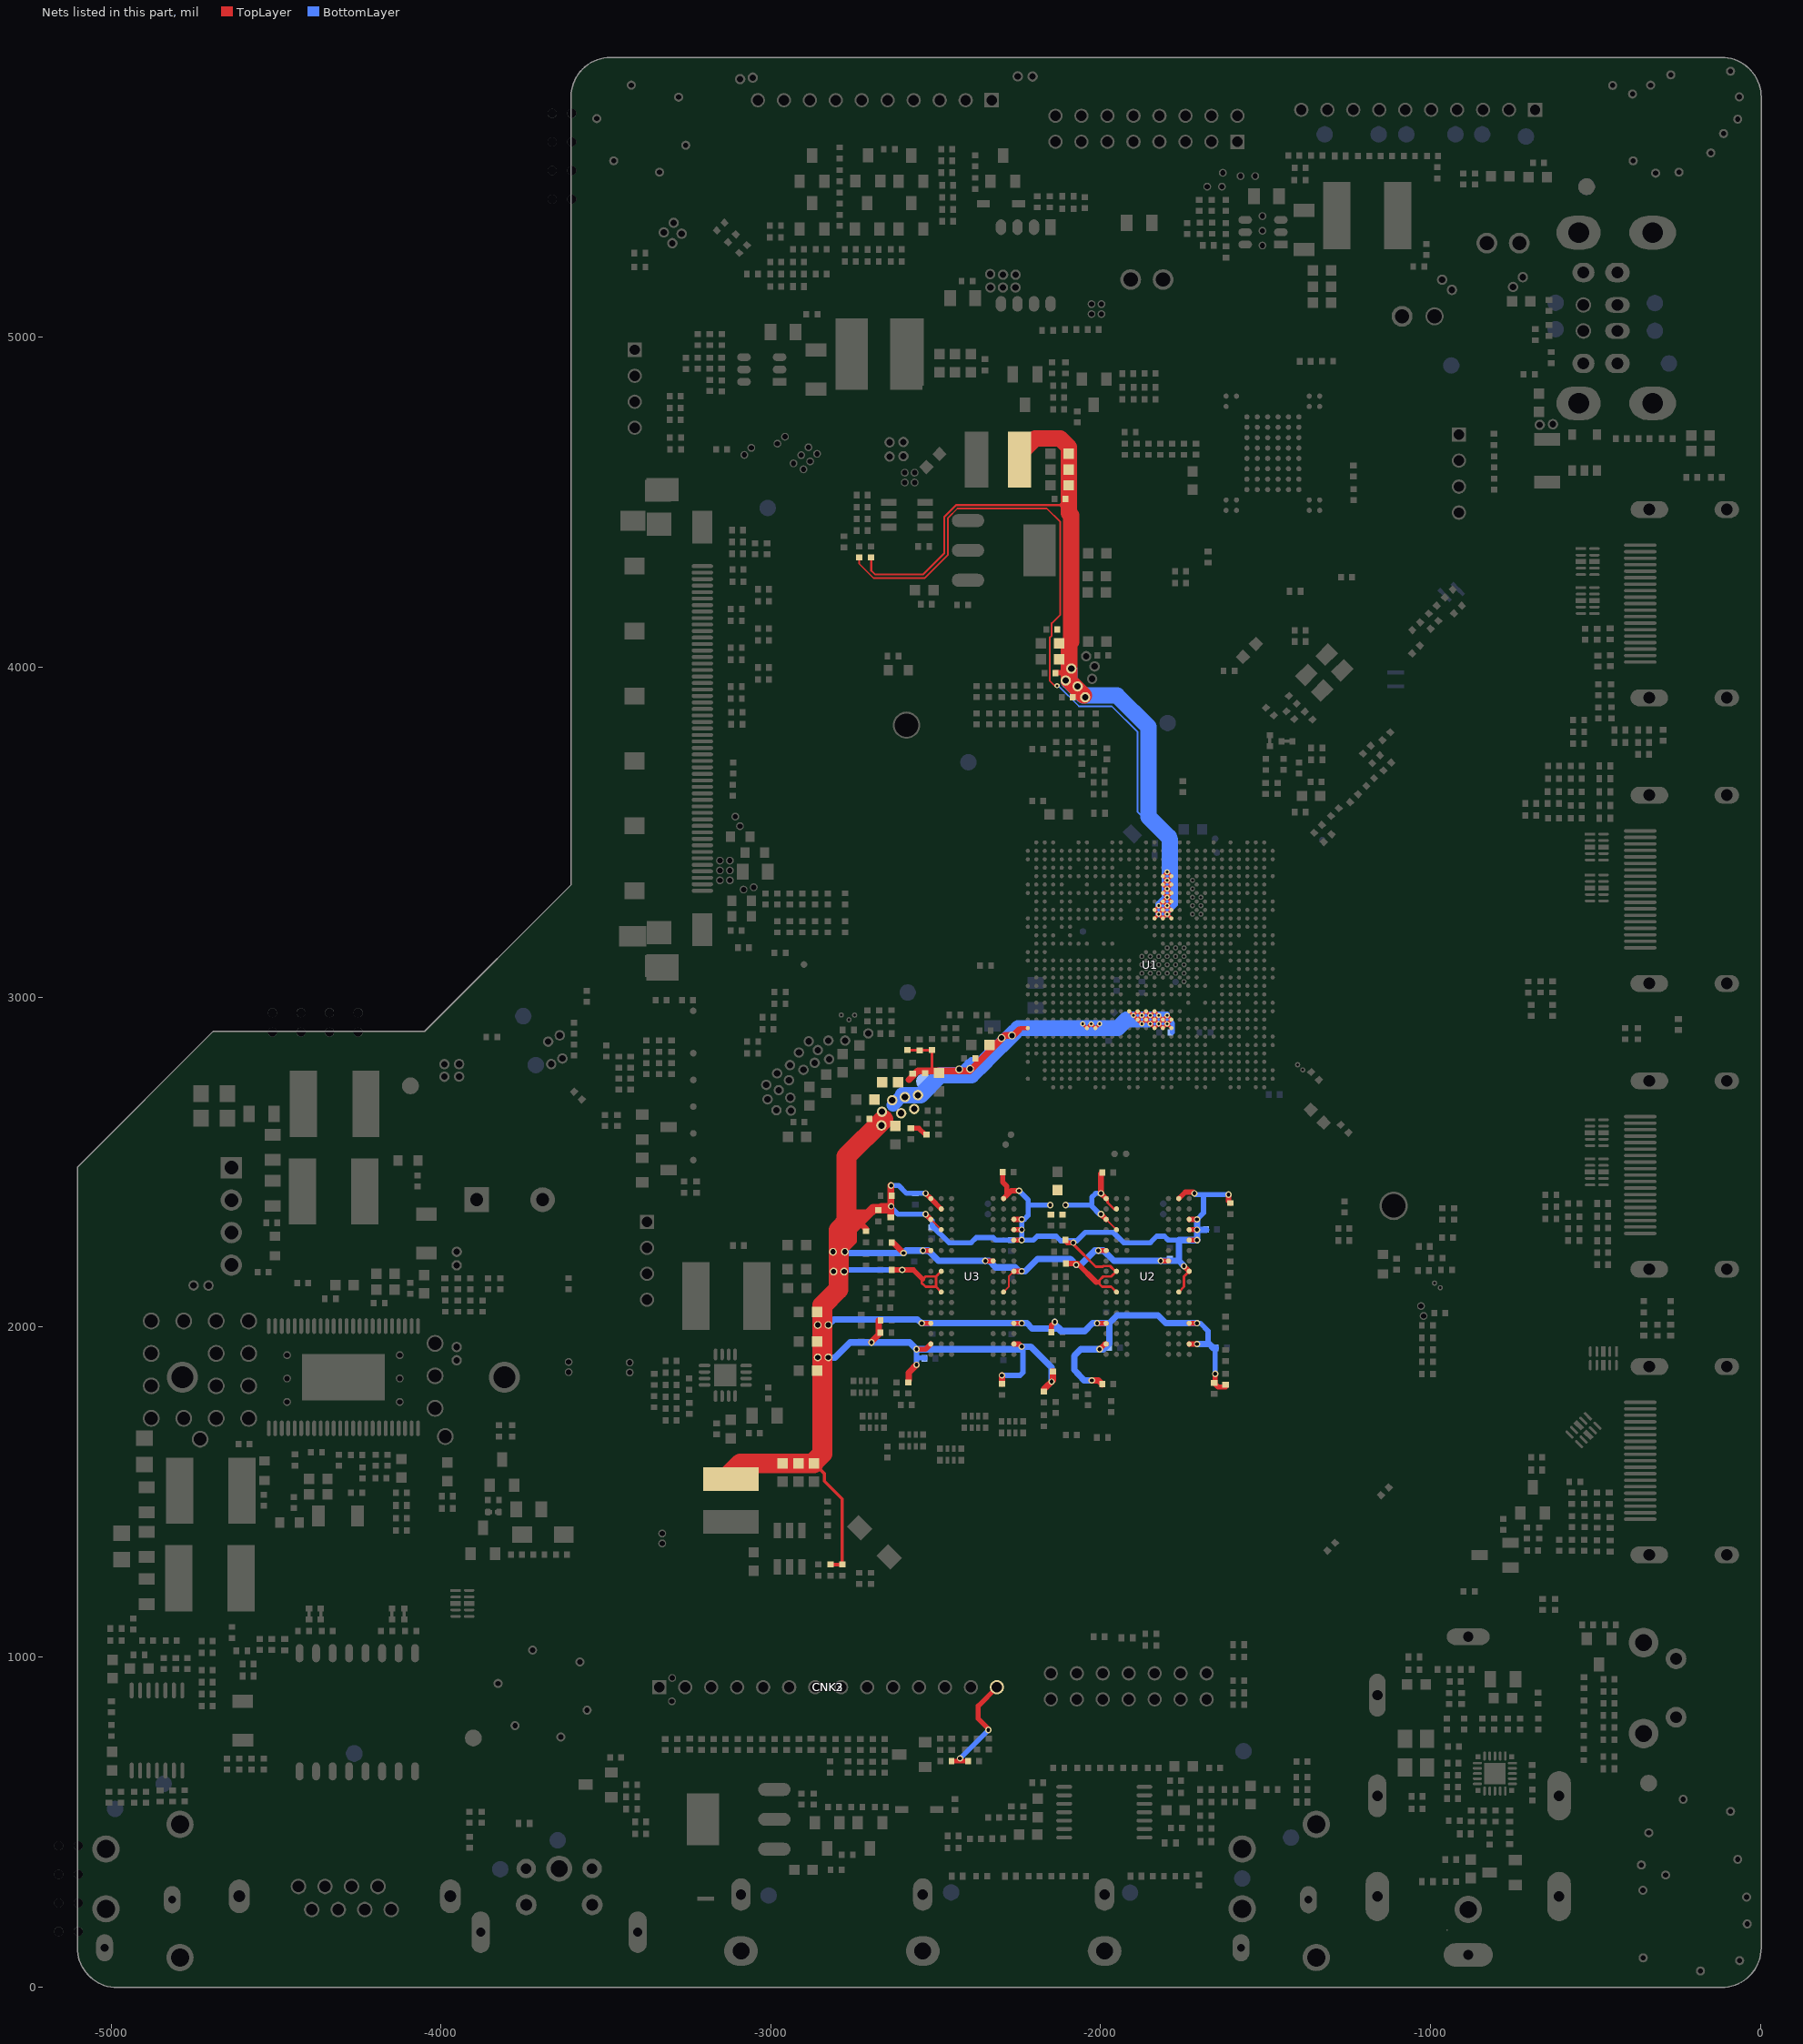
[diagram p0: the nets of this part, all layers, seen from the top]
# Altium PCB MISC86290.PcbDoc (part 8 of 31)
Units mil, origin at the board's own origin, x right, y up, seen from the top; angles counter-clockwise.
Board outline 5104.71 x 5851.49 mil, 2 copper layers (TopLayer, BottomLayer), stack 61.855 mil thick; 1026 components, 667 nets, 4280 pads, 2294 vias.

## Via types
v1: diameter 19.68, hole 11.81, TopLayer to BottomLayer, tented both sides, 1189 vias
v2: diameter 19.68/19.68 (per signal layer), hole 11.81, TopLayer to BottomLayer, tented both sides, 366 vias
v3: diameter 15.75, hole 7.87, TopLayer to BottomLayer, tented both sides, 348 vias
v4: diameter 23.62, hole 15.75, TopLayer to BottomLayer, tented both sides, 309 vias
v5: diameter 15.75/15.75 (per signal layer), hole 7.87, TopLayer to BottomLayer, tented both sides, 59 vias
v6: diameter 24/24 (per signal layer), hole 16, TopLayer to BottomLayer, tented both sides, 23 vias

## Nets (pads, with @x,y where several pads share a name; then routed paths per layer and width w, separated by ;. In a path a pad name is that pad's centre, name@x,y a point inside that pad or via, vN(x,y) a via of type N, cw(c..) or ccw(c..) an arc to the next point about the centre after c; other vN are vias at no path point) (continued)
0.95V_VDDCPU: C32.1 C33.1 C34.1 C35.2 C36.2 C209.1 C210.1 C211.1 CD53.2 CD54.2 CD55.2 CD56.2 LD51.2 pad.VIA5@-1798.54,3251.57 pad.VIA5@-1798.54,3277.17 pad.VIA5@-1798.54,3302.76 pad.VIA5@-1798.54,3328.35 pad.VIA5@-1798.54,3353.94 pad.VIA5@-1798.54,3379.53 pad.VIA5@-1824.13,3251.57 pad.VIA5@-1824.13,3277.17 pad.VIA5@-2047,3909 pad.VIA5@-2070,3942 pad.VIA5@-2089,3996 pad.VIA5@-2106,3960 RD53.2 RD60.1 U1.AA13 U1.AA14 U1.AA15 U1.AB13 U1.AB14 U1.AB15 U1.AC13 U1.AC14 U1.AD13 U1.AD14 U1.AE13 U1.AE14 U1.AF13 U1.AF14 | length 5527.1
  TopLayer w5: RD60.1@-2732.5,4333.04 -2732.5,4314.54 -2687.96,4270 -2534.42,4270 -2463,4341.42 -2463,4452.69 -2434.26,4481.43 -2163.43,4481.43 -2122.5,4440.5 -2122.5,4159.5 -2148.46,4133.54 -2148.46,4096.54 -2154,4091 -2154,3958 v3@-2140,3944
  TopLayer w6: RD53.2@-2695.5,4333.04 -2695.5,4293 -2683.5,4281 -2539.3,4281 -2474.4,4345.9 -2474.4,4456.02 -2438.64,4491.78 -2123.99,4491.78 ; CD53.2@-2101.91,4504.86 -2096.84,4509.92 ; CD53.2@-2101.91,4513.86 -2123.99,4491.78 ; -2096.84,4464.63 -2123.99,4491.78
  TopLayer w10: U1.AA15@-1836.93,3238.78 pad.VIA5@-1824.13,3251.57 ; U1.AA13@-1785.75,3238.78 pad.VIA5@-1798.54,3251.57 ; pad.VIA5@-1824.13,3251.57 U1.AB15@-1836.93,3264.37 pad.VIA5@-1824.13,3277.17 ; pad.VIA5@-1824.13,3251.57 U1.AA14@-1811.34,3238.78 pad.VIA5@-1798.54,3251.57 ; pad.VIA5@-1824.13,3251.57 U1.AB14@-1811.34,3264.37 ; pad.VIA5@-1824.13,3277.17 U1.AB14@-1811.34,3264.37 ; pad.VIA5@-1824.13,3277.17 U1.AC14@-1811.34,3289.96 ; U1.AB14@-1811.34,3264.37 pad.VIA5@-1798.54,3251.57 ; U1.AB14@-1811.34,3264.37 pad.VIA5@-1798.54,3277.17 ; U1.AC14@-1811.34,3289.96 pad.VIA5@-1798.54,3277.17 ; U1.AC14@-1811.34,3289.96 pad.VIA5@-1798.54,3302.76 ; pad.VIA5@-1798.54,3251.57 U1.AB13@-1785.75,3264.37 pad.VIA5@-1798.54,3277.17 ; pad.VIA5@-1798.54,3277.17 U1.AC13@-1785.75,3289.96 pad.VIA5@-1798.54,3302.76 ; pad.VIA5@-1798.54,3302.76 U1.AD13@-1785.75,3315.55 pad.VIA5@-1798.54,3328.35 ; pad.VIA5@-1798.54,3302.76 U1.AD14@-1811.34,3315.55 pad.VIA5@-1798.54,3328.35 ; pad.VIA5@-1798.54,3328.35 U1.AE13@-1785.75,3341.14 pad.VIA5@-1798.54,3353.94 ; pad.VIA5@-1798.54,3328.35 U1.AE14@-1811.34,3341.14 pad.VIA5@-1798.54,3353.94 ; pad.VIA5@-1798.54,3353.94 U1.AF13@-1785.75,3366.73 pad.VIA5@-1798.54,3379.53 U1.AF14@-1811.34,3366.73 pad.VIA5@-1798.54,3353.94
  TopLayer w17: C33.1@-2137.27,3984 -2120.45,3984 ; pad.VIA5@-2076.68,3941.77 pad.VIA5@-2066.23,3941.77
  TopLayer w50: LD51.2@-2246.24,4629.43 -2246.24,4645.79 -2198.03,4694 -2123,4694 -2096.84,4667.84 -2096.84,4509.92 -2096.84,4467.84 -2089.83,4460.83 -2089.83,4077.92 ; -2095.75,4072 -2095.75,3959.3 -2077.45,3941 -2074.23,3937.77 pad.VIA5@-2051.45,3915
  BottomLayer w5: v3@-2128.5,3944 -2066,3881.5 -1966.23,3881.5 -1888,3803.27 -1888,3561.28 -1875.62,3548.89 ; pad.VIA5@-1799.72,3278.03 pad.VIA5@-1799.27,3278.03
  BottomLayer w12: pad.VIA5@-1824.13,3254.03 -1822.93,3255.24 -1822.93,3277.17 -1822.93,3278.03 pad.VIA5@-1823.1,3278.2 ; pad.VIA5@-1800.13,3278.03 pad.VIA5@-1799.72,3278.03 ; pad.VIA5@-1799.27,3278.03 pad.VIA5@-1797.72,3278.03
  BottomLayer w15: pad.VIA5@-1798.54,3328.35 -1797.72,3327.53 -1797.72,3324.03 -1790.72,3324.03 -1773.22,3324.03 -1773.22,3281.03 -1794.72,3259.53
  BottomLayer w18: pad.VIA5@-1824.13,3251.57 pad.VIA5@-1799.72,3275.98 ; -1806.14,3299.12 pad.VIA5@-1806.14,3302.03 ; pad.VIA5@-1798.54,3379.53 -1806.14,3379.53 pad.VIA5@-1806.14,3302.03 ; pad.VIA5@-1793.68,3282.03 pad.VIA5@-1798.54,3277.17 pad.VIA5@-1799.72,3275.98 ; pad.VIA5@-1806.14,3302.03 -1799.72,3295.62 -1799.72,3278.03 -1799.72,3277.17 pad.VIA5@-1799.72,3275.98
  BottomLayer w20: pad.VIA5@-1823.1,3278.2 pad.VIA5@-1824.13,3277.17 ; -1806.14,3299.12 -1824.13,3281.12 pad.VIA5@-1824.13,3277.17 ; pad.VIA5@-1798.54,3251.57 pad.VIA5@-1824.13,3251.57 -1824.13,3254.03 pad.VIA5@-1824.13,3277.17 ; pad.VIA5@-1798.54,3277.17 -1799.72,3277.17 -1822.93,3277.17 pad.VIA5@-1824.13,3277.17
  BottomLayer w50: pad.VIA5@-2095.75,3995 -2095.75,3957.75 -2053,3915 -1951,3915 -1855,3819 -1855,3546.69 -1793.37,3485.06 ; -1790.72,3294.53 -1790.72,3324.03 -1790.72,3477.39
  other v3: -2132.5,3944
1V5_DDR: 1V5_DDR.1 C37.1 C38.1 C39.2 C40.2 C41.2 C42.1 C43.1 C44.2 C45.1 C46.2 C48.1 C50.1 C51.2 C58.2 C61.2 C62.2 C63.2 C64.2 C65.2 C66.2 C67.2 C68.2 C69.2 C70.2 C71.2 C73.2 C74.2 C75.2 C76.2 C77.2 C78.2 C79.2 C80.2 C81.2 C82.2 C83.2 C84.2 C85.2 C86.2 C87.2 C88.2 C89.2 C90.2 C91.2 C92.2 C93.2 C94.2 C95.2 C96.2 C206.1 C207.1 C208.1 CD23.2 CD25.2 CD26.2 CD27.2 LD21.2 pad.VIA5@-1798.54,2918.9 pad.VIA5@-1798.54,2944.49 pad.VIA5@-1824.13,2918.9 pad.VIA5@-1824.13,2944.49 pad.VIA5@-1849.72,2918.9 pad.VIA5@-1849.72,2944.49 pad.VIA5@-1875.32,2918.9 pad.VIA5@-1875.32,2944.49 pad.VIA5@-1900.91,2944.49 pad.VIA5@-2003.27,2918.9 pad.VIA5@-2028.86,2918.9 pad.VIA5@-2054.45,2918.9 pad.VIA5@-2269.02,2883.46 pad.VIA5@-2300.6,2876.14 pad.VIA5@-2396.1,2782.4 pad.VIA5@-2429,2781 pad.VIA5@-2554,2703.03 pad.VIA5@-2565.5,2661 pad.VIA5@-2593.5,2697 pad.VIA5@-2605,2648 pad.VIA5@-2632,2687.5 pad.VIA5@-2663,2652.5 pad.VIA5@-2665,2611 pad.VIA5@-2775.72,2228.03 pad.VIA5@-2777.72,2168.03 pad.VIA5@-2809.72,2168.03 pad.VIA5@-2811.72,2228.03 pad.VIA5@-2825.72,1908.03 pad.VIA5@-2825.72,2006.03 pad.VIA5@-2857.72,1908.03 pad.VIA5@-2857.72,2006.03 R44.2 R46.2 R63.2 R66.2 R101.2 R103.2 R107.2 R118.2 RD22.2 U1.H13 U1.H14 U1.H15 U1.H22 U1.H23 U1.H30 U1.J13 U1.J14 U1.J15 U1.J16 U1.J17 U1.K15 U1.K16 U1.K17 U1.K18 U2.A1 U2.A8 U2.B2 U2.C1 U2.C9 U2.D2 U2.D9 U2.E9 U2.F1 U2.G7 U2.H2 U2.H9 U2.K2 U2.K8 U2.N1 U2.N9 U2.R1 U2.R9 U3.A1 U3.A8 U3.B2 U3.C1 U3.C9 U3.D2 U3.D9 U3.E9 U3.F1 U3.G7 U3.H2 U3.H9 U3.K2 U3.K8 U3.N1 U3.N9 U3.R1 U3.R9 | length 13478.8
  TopLayer w3.94: U3.C1@-2515.08,2326.38 U3.D2@-2483.58,2294.88 ; U2.C1@-1983.58,2326.38 U2.D2@-1952.09,2294.88
  TopLayer w5: CD23.2@-2783.52,1279.73 CD23.2@-2783.25,1280 ; -2539.72,2144.25 -2539.43,2144.54 ; pad.VIA5@-2269.02,2883.46 pad.VIA5@-2269.02,2883.86 ; C82.2@-2107.28,2263.78 -2107.28,2261.42 C82.2@-2106.83,2260.96
  TopLayer w5.91: U3.K8@-2294.61,2105.91 -2278.86,2121.65 -2278.86,2153.15 U3.H9@-2263.11,2168.9
  TopLayer w7.87: -2539.72,2144.25 -2542.64,2141.34 -2542.64,2133.46 -2530.83,2121.65 -2499.33,2121.65 ; -2539.43,2144.54 -2530.83,2153.15 -2499.33,2153.15 ; U3.K2@-2483.58,2105.91 -2499.33,2121.65 ; U3.H2@-2483.58,2168.9 -2499.33,2153.15 ; v2(-2082.99,2255.51) -2082.01,2249.61 -2015.08,2182.68 -1993.43,2182.68 -1991.46,2184.65 -1971.77,2184.65 -1956.02,2168.9 U2.H2@-1952.09,2168.9 -1967.83,2153.15 -1992.44,2153.15 -2004.25,2141.34 -2004.25,2135.43 ; -2013.11,2135.43 -2004.25,2135.43 ; U2.A1@-1983.58,2389.37 -1979.65,2385.43 -1979.65,2377.56 -1959.96,2357.87 U2.B2@-1952.09,2357.87 ; U2.K2@-1952.09,2105.91 -1967.83,2121.65 -1995.39,2121.65 -2004.25,2130.51 -2004.25,2135.43 ; U2.K8@-1763.11,2105.91 -1747.36,2121.65 -1747.36,2153.15 U2.H9@-1731.61,2168.9 ; -2499.33,2121.65 -2499.33,2153.15
  TopLayer w8: C38.1@-2585.66,2839.58 R46.2@-2511.84,2839.58 -2511.84,2776.03 -2511.84,2775.6
  TopLayer w9.84: U1.H14@-1812.32,2907.09 U1.H14@-1811.34,2906.1 pad.VIA5@-1798.54,2918.9 U1.J13@-1785.75,2931.69
  TopLayer w10: CD27.2@-2869.29,1586.68 -2838,1555.4 -2838,1533 -2783.52,1478.52 CD23.2@-2783.52,1279.73 ; RD22.2@-2819.25,1279.73 CD23.2@-2783.52,1279.73 ; CD23.2@-2783.52,1278.74 CD23.2@-2783.52,1279.73 ; pad.VIA5@-2054.45,2918.9 U1.H23@-2041.65,2906.1 pad.VIA5@-2028.86,2918.9 U1.H22@-2016.06,2906.1 pad.VIA5@-2003.27,2918.9 ; U1.K18@-1913.7,2957.28 pad.VIA5@-1900.91,2944.49 ; U1.H14@-1812.32,2907.09 pad.VIA5@-1824.13,2918.9 ; U1.H13@-1785.75,2906.1 pad.VIA5@-1798.54,2918.9 -1806.2,2926.56 U1.J14@-1811.34,2931.69 ; U1.J13@-1785.75,2931.69 pad.VIA5@-1798.54,2944.49 U1.J14@-1811.34,2931.69 ; pad.VIA5@-1900.91,2944.49 U1.J17@-1888.11,2931.69 ; pad.VIA5@-1900.91,2944.49 U1.K17@-1888.11,2957.28 pad.VIA5@-1875.32,2944.49 ; U1.J17@-1888.11,2931.69 pad.VIA5@-1875.32,2944.49 ; U1.J17@-1888.11,2931.69 pad.VIA5@-1875.32,2918.9 U1.J16@-1862.52,2931.69 ; pad.VIA5@-1875.32,2944.49 U1.J16@-1862.52,2931.69 ; pad.VIA5@-1875.32,2944.49 U1.K16@-1862.52,2957.28 pad.VIA5@-1849.72,2944.49 ; U1.J16@-1862.52,2931.69 pad.VIA5@-1849.72,2944.49 ; U1.J16@-1862.52,2931.69 pad.VIA5@-1849.72,2918.9 ; pad.VIA5@-1849.72,2918.9 U1.H15@-1836.93,2906.1 pad.VIA5@-1824.13,2918.9 ; pad.VIA5@-1849.72,2918.9 U1.J15@-1836.93,2931.69 ; pad.VIA5@-1849.72,2944.49 U1.K15@-1836.93,2957.28 pad.VIA5@-1824.13,2944.49 ; pad.VIA5@-1849.72,2944.49 U1.J15@-1836.93,2931.69 ; U1.J15@-1836.93,2931.69 pad.VIA5@-1824.13,2918.9 ; U1.J15@-1836.93,2931.69 pad.VIA5@-1824.13,2944.49 ; pad.VIA5@-1824.13,2918.9 U1.J14@-1811.34,2931.69 ; pad.VIA5@-1824.13,2944.49 U1.J14@-1811.34,2931.69
  TopLayer w12: -2248.33,2900.43 -2242.65,2906.1 U1.H30@-2220.79,2906.1
  TopLayer w15: C77.2@-2575.5,2602.46 -2550.84,2602.46 -2531.41,2583.04 C48.1@-2528.5,2583.04
  TopLayer w15.75: C68.2@-2634.12,2172.83 v2(-2601.69,2172.83) -2567.72,2172.83 -2539.43,2144.54 ; v2(-2558.39,1932.68) -2530.83,1932.68 U3.R1@-2515.08,1948.43 ; v2(-2542.64,2011.42) U3.N1@-2515.08,2011.42 ; v2(-2538.7,2231.89) U3.F1@-2515.08,2231.89 ; v2(-2530.83,2342.13) U3.C1@-2515.08,2326.38 ; v2(-2530.83,2405.12) U3.A1@-2515.08,2389.37 U3.B2@-2483.58,2357.87 ; v2(-2349.72,2200.39) U3.G7@-2326.1,2200.39 ; C76.2@-2296.89,2470.08 -2296.97,2470 -2296.97,2438.98 -2284.76,2426.77 -2284.76,2399.21 ; U3.A8@-2294.61,2389.37 -2284.76,2399.21 ; U3.R9@-2263.11,1948.43 -2247.36,1948.43 v2(-2239.49,1940.55) ; U3.N9@-2263.11,2011.42 v2(-2239.49,2011.42) ; U3.H9@-2263.11,2168.9 v2(-2239.49,2168.9) ; U3.E9@-2263.11,2263.39 v2(-2239.49,2263.39) ; U3.D9@-2263.11,2294.88 v2(-2239.49,2294.88) ; U3.C9@-2263.11,2326.38 v2(-2239.49,2326.38) ; v2(-2247.36,2412.99) -2270.98,2412.99 -2284.76,2399.21 ; C81.2@-2149.25,1983.86 -2149.25,2005.2 v2(-2139.09,2015.35) ; C82.2@-2106.83,2260.96 -2101.38,2255.51 v2(-2082.99,2255.51) ; C73.2@-2105.32,2192.52 -2070.2,2192.52 -2013.11,2135.43 ; v2(-2011.14,2011.42) U2.N1@-1983.58,2011.42 ; v2(-2007.2,2231.89) U2.F1@-1983.58,2231.89 ; v2(-2003.27,1932.68) -1987.52,1948.43 U2.R1@-1983.58,1948.43 ; v2(-1999.33,2342.13) U2.C1@-1983.58,2326.38 ; v2(-1999.33,2405.12) U2.A1@-1983.58,2389.37 ; v2(-1818.23,2200.39) U2.G7@-1794.61,2200.39 ; U2.A8@-1763.11,2389.37 -1743.43,2409.06 -1719.8,2409.06 v2(-1715.87,2405.12) ; v2(-1747.36,2184.65) U2.H9@-1731.61,2168.9 ; U2.R9@-1731.61,1948.43 v2(-1707.99,1948.43) ; U2.N9@-1731.61,2011.42 v2(-1707.99,2011.42) ; U2.E9@-1731.61,2263.39 v2(-1707.99,2263.39) ; U2.D9@-1731.61,2294.88 v2(-1707.99,2294.88) ; U2.C9@-1731.61,2326.38 v2(-1707.99,2326.38) ; v2(-1652.87,1857.87) -1652.87,1832.6 -1654.84,1830.63 -1654.84,1828.66 -1644.37,1818.19 R66.2@-1621.38,1818.19 ; v2(-1612.52,2401.18) -1612.52,2381.81 C70.2@-1606.61,2375.91
  TopLayer w17.72: v2(-1999.33,2405.12) -1999.33,2464.49 C67.2@-1995.71,2468.11
  TopLayer w18: C69.2@-2629.25,2255.51 v2(-2597.76,2224.02)
  TopLayer w19.68: v2(-2694.72,1953.03) -2694.72,1955.53 -2672.87,1977.38 R101.2@-2672.87,2019.29 ; C79.2@-2636.41,2334.57 -2636.41,2353.94 ; v2@-2636.41,2428.74 v2@-2636.41,2365.75 ; R107.2@-2582.01,1838.5 -2582.01,1861.81 v2(-2558.39,1885.43) ; C50.1@-2299.53,1828.07 v2(-2299.53,1852.95) ; R118.2@-2172.56,1810.94 -2164.84,1818.66 -2164.53,1818.66 v2(-2148.94,1834.25) -2145,1838.19 C42.1@-2145,1865.43 ; v2(-2026.89,1838.19) -2007.2,1838.19 R63.2@-1995.39,1826.69 R63.2@-1995.71,1826.38 ; -2636.41,2353.94 v2@-2636.41,2365.75 ; -2636.41,2353.94 -2669.56,2353.94 -2671.87,2356.25 -2673.81,2358.19 -2666.25,2365.75 v2@-2636.41,2365.75
  TopLayer w20: C61.2@-2854.97,1860.03 -2843.47,1859.75 ; C63.2@-2854.97,1958.03 -2843.47,1954.63 ; C62.2@-2854.97,2058.03 -2851.42,2054.94 -2843.47,2048.03 ; -2843.47,1908.03 pad.VIA5@-2826.97,1908.03 ; -2843.47,2006.03 pad.VIA5@-2826.97,2006.03 ; pad.VIA5@-2810.97,2168.03 -2810.97,2166.03 -2794.97,2150.03 ; -2730.89,2316.85 R103.2@-2711.21,2297.16 ; -2580.97,2749.72 -2561.55,2769.14 -2554.66,2776.03 ; -2553.41,2776.03 -2511.84,2776.03 -2397.72,2776.03 pad.VIA5@-2393.72,2780.03 ; pad.VIA5@-2396.1,2782.4 pad.VIA5@-2393.72,2780.03 ; -2248.33,2900.43 -2264.9,2883.86 -2269.02,2883.86 -2289.9,2883.86 pad.VIA5@-2393.72,2780.03
  TopLayer w29.53: pad.VIA5@-2778.97,2168.03 -2778.97,2236.9 -2753.47,2262.4 -2753.47,2294.27 -2730.89,2316.85 -2706.34,2341.4 ; -2770.97,2341.4 -2706.34,2341.4 ; C71.2@-2673.81,2358.19 -2689.56,2358.19 -2706.34,2341.4
  TopLayer w60: LD21.2@-3124.25,1554.87 -3092.44,1586.68 CD25.2@-2963.9,1586.68 CD26.2@-2916.59,1586.68 CD27.2@-2869.29,1586.68 ; CD27.2@-2869.29,1590.37 -2843.47,1616.18 -2843.47,1830.88 ; -2843.74,1830.62 -2843.47,1830.88 ; -2658.5,2629 -2770.97,2516.53 -2770.97,2341.4 -2770.97,2318.03 -2794.97,2294.03 -2794.97,2150.03 -2794.97,2114.03 -2843.47,2065.53 -2843.47,2048.03 -2843.47,2006.03 -2843.47,1954.63 -2843.47,1908.03 -2843.47,1859.75 -2843.47,1830.88
  BottomLayer w5: pad.VIA5@-2777.72,2168.03 pad.VIA5@-2777.72,2173.03 ; C89.2@-2568.23,2232.2 C89.2@-2566.41,2232.2 ; C89.2@-2566.72,2231.89 C89.2@-2566.41,2232.2 ; C89.2@-2566.26,2232.2 C89.2@-2566.41,2232.2 ; C84.2@-2513.72,2306.01 -2510.74,2306.01 C84.2@-2510.6,2306.15 ; C86.2@-2511.14,2011.42 C86.2@-2511.14,2011.73 ; C83.2@-2294.61,1932.68 C83.2@-2294.61,1932.99 ; C91.2@-2270.98,2011.73 -2270.04,2011.73 C91.2@-2269.72,2011.42 ; C93.2@-2270.98,2180.71 C93.2@-2270.98,2182.99 ; C92.2@-2270.98,2263.39 C92.2@-2270.98,2266.65 ; C96.2@-1980.63,2010.12 C96.2@-1980.63,2011.42 ; C95.2@-1788.7,2199.59 -1788.7,2199.87 C95.2@-1788.18,2200.39
  BottomLayer w9.84: -1793.96,2932.03 -1792.32,2930.39
  BottomLayer w15.75: pad.VIA5@-2809.72,2168.03 -2804.72,2173.03 -2777.72,2173.03 -2601.69,2173.03 v2(-2601.69,2172.83) ; v2(-2635.16,2365.75) -2635.16,2362.13 -2615.16,2342.13 v2(-2530.83,2342.13) -2511.14,2322.44 -2511.14,2306.69 -2510.6,2306.15 -2459.96,2255.51 -2393.03,2255.51 -2377.28,2271.26 -2326.1,2271.26 -2318.23,2263.39 C92.2@-2270.98,2263.39 v2(-2239.49,2263.39) ; v2(-2635.16,2428.74) -2612.43,2428.74 -2588.81,2405.12 v2(-2530.83,2405.12) ; v2(-2558.39,1885.43) v2(-2558.39,1932.68) v2@-2554.45,1932.68 ; -2558.39,1906.03 -2533.11,1906.03 C94.2@-2533.11,1905.12 ; v2(-2299.53,1852.95) -2244.63,1852.95 -2235.55,1862.03 v2@-2235.55,1940.55 ; v2(-2247.36,2412.99) -2219.8,2385.43 -2219.8,2369.69 ; v2(-2152.87,2369.69) -2219.8,2369.69 ; v2(-2106.61,2369.69) -2026.89,2369.69 ; v2(-2082.99,2255.51) v2@-2085.94,2261.42 ; v2(-1999.33,2342.13) -2003.27,2342.13 -2026.89,2365.75 -2026.89,2369.69 ; v2(-1999.33,2405.12) -2015.08,2405.12 -2026.89,2393.31 -2026.89,2369.69 ; pad.VIA5@-1900.91,2944.49 pad.VIA5@-1875.32,2944.49 -1863.92,2944.49 -1860.28,2948.13 -1798.54,2948.13 pad.VIA5@-1798.54,2944.49 pad.VIA5@-1798.54,2937.1 ; -1792.32,2930.39 -1786.49,2924.56 ; -1763.11,2263.39 -1795.08,2263.39 -1806.89,2275.2 -1830.04,2275.2 -1849.72,2255.51 -1930.43,2255.51 -1961.93,2287.01 -2046.57,2287.01 -2072.17,2261.42 v2@-2085.94,2261.42 ; v2(-1715.87,2405.12) -1711.93,2401.18 -1688.31,2401.18 ; v2(-1707.99,2011.42) -1698.15,2011.42 -1674.53,1987.8 -1674.53,1948.43 ; v2(-1707.99,2326.38) -1688.31,2346.06 -1688.31,2401.18 ; v2(-1652.87,1857.87) C88.2@-1652.87,1936.61 ; v2(-1612.52,2401.18) -1688.31,2401.18 ; v2(-2239.49,2263.39) v2(-2239.49,2294.88) v2(-2239.49,2326.38) -2231.61,2326.38 -2219.8,2338.19 -2219.8,2369.69 ; v2(-2239.49,2263.39) -2204.06,2263.39 -2192.24,2275.2 -2135.16,2275.2 -2121.38,2261.42 v2@-2085.94,2261.42 ; pad.VIA5@-1798.54,2937.1 -1786.49,2925.04 -1786.49,2924.56 ; pad.VIA5@-1798.54,2937.1 -1798.54,2932.03 pad.VIA5@-1798.54,2918.9 -1792.64,2918.9 -1782.8,2909.06 -1782.48,2893.44 -1782.48,2893.31 -1782.48,2920.55 -1786.49,2924.56
  BottomLayer w19.68: pad.VIA5@-2825.72,1908.03 -2824.77,1907.07 -2805.72,1907.07 -2759.72,1953.07 -2679.73,1953.07 ; pad.VIA5@-2825.72,2006.03 -2808.72,2023.03 -2556.42,2023.03 v2(-2542.64,2011.42) -2511.14,2011.42 C91.2@-2269.72,2011.42 v2(-2239.49,2011.42) -2223.74,2011.42 -2207.99,1995.67 -2152.87,1995.67 ; pad.VIA5@-2811.72,2228.03 -2807.72,2224.02 pad.VIA5@-2773.72,2224.02 ; pad.VIA5@-2775.72,2228.03 -2773.72,2226.03 pad.VIA5@-2773.72,2224.02 ; v2(-2694.72,1953.03) -2679.73,1953.07 ; v2(-2558.39,1932.68) -2579.06,1953.35 -2679.73,1953.07 ; v2@-2554.45,1932.68 -2294.61,1932.68 -2247.36,1932.68 v2(-2239.49,1940.55) -2235.55,1940.55 -2211.93,1940.55 -2148.94,1877.56 v2(-2148.94,1834.25) ; v2(-2139.09,2015.35) v2@-2139.09,2009.45 ; v2(-2026.89,1838.19) -2050.51,1838.19 -2080.04,1869.69 -2080.04,1912.99 -2060.35,1932.68 v2(-2003.27,1932.68) -1991.46,1932.68 -1973.74,1950.39 -1973.74,2011.42 ; -1855.63,2932.03 -1825.46,2932.03 ; pad.VIA5@-1849.72,2918.9 pad.VIA5@-1824.13,2918.9 -1812.32,2918.9 ; pad.VIA5@-1798.54,2918.9 -1812.32,2918.9 ; -1798.54,2932.03 -1825.46,2932.03 ; v2(-1747.36,2184.65) -1763.11,2200.39 ; v2(-1707.99,1948.43) -1674.53,1948.43 ; v2(-1707.99,2011.42) -1802.48,2011.42 -1826.1,2035.04 -1950.12,2035.04 -1973.74,2011.42 ; v2(-1707.99,2326.38) v2(-1707.99,2294.88) ; C85.2@-1680.75,2294.88 v2(-1707.99,2294.88) ; pad.VIA5@-2773.72,2224.02 v2(-2597.76,2224.02) -2589.88,2231.89 -2566.72,2231.89 v2(-2538.7,2231.89) -2522.95,2231.89 -2491.46,2200.39 v2(-2349.72,2200.39) -2337.91,2200.39 -2318.23,2180.71 C93.2@-2270.98,2180.71 -2259.4,2180.71 -2247.59,2168.9 v2(-2239.49,2168.9) -2228.66,2168.9 -2191.26,2206.3 -2091.85,2206.3 v2(-2074.13,2188.58) -2061.34,2188.58 -2018.03,2231.89 v2(-2007.2,2231.89) -1991.46,2231.89 -1959.96,2200.39 v2(-1818.23,2200.39) -1788.18,2200.39 -1763.11,2200.39 ; -2152.87,1995.67 -2145,1995.67 ; -2152.87,1995.67 v2@-2139.09,2009.45 ; -2145,1995.67 -2129.72,1995.67 -2129.49,1995.91 -2121.38,1987.8 ; -2145,1995.67 -2139.09,2003.54 v2@-2139.09,2009.45 ; v2@-2139.09,2009.45 -2121.38,1991.73 -2121.38,1987.8 ; -2121.38,1987.8 -2048.54,1987.8 -2024.92,2011.42 v2(-2011.14,2011.42) C96.2@-1983.58,2011.42 -1980.63,2011.42 -1973.74,2011.42 ; -1825.46,2932.03 -1818.23,2924.8 -1812.32,2918.9 ; -1763.11,2200.39 -1763.11,2263.39 v2(-1707.99,2263.39) v2(-1707.99,2294.88)
  BottomLayer w20: pad.VIA5@-2857.72,1908.03 pad.VIA5@-2825.72,1908.03 ; pad.VIA5@-2857.72,2006.03 pad.VIA5@-2825.72,2006.03 ; -2054.45,2905.53 pad.VIA5@-2054.45,2918.9 ; -1674.53,1948.43 -1670.59,1948.43 -1658.78,1936.61 -1652.87,1936.61 C88.2@-1651.22,1936.61
  BottomLayer w24: -2437.22,2763.03 -2400.97,2799.28 -2398.47,2799.28 ; -2405.72,2792.03 -2398.47,2799.28 ; -2348.22,2807.03 -2349.22,2806.03 -2391.72,2806.03 -2398.47,2799.28
  BottomLayer w40: pad.VIA5@-2629.5,2673.5 pad.VIA5@-2599.97,2703.03
  BottomLayer w48: -2260.6,2894.66 -2249.72,2905.53 -2054.45,2905.53 -1948.22,2905.53 -1921.72,2932.03 -1855.63,2932.03
  BottomLayer w50: pad.VIA5@-2599.97,2703.03 pad.VIA5@-2554,2703.03 -2545.97,2703.03 -2485.97,2763.03 ; -2484.72,2763.03 -2437.22,2763.03 -2392.22,2763.03 -2349.22,2806.03 ; -2348.22,2807.03 -2260.6,2894.66
3V3_IR: CK8.2 CNK2.14 CNK3.14 RK23.2 | length 350.1
  TopLayer w15: RK23.2@-2452.27,684 -2434.83,684 ; v1(-2426.43,692.4) -2434.83,684 ; CK8.2@-2401.73,684 -2434.83,684 ; v1(-2340.5,778.5) -2340.5,781.52 -2371.5,812.52 -2371.5,851 CNK2.14@-2314.5,908
  BottomLayer w15: v1(-2426.43,692.4) -2340.5,778.33 v1(-2340.5,778.5)